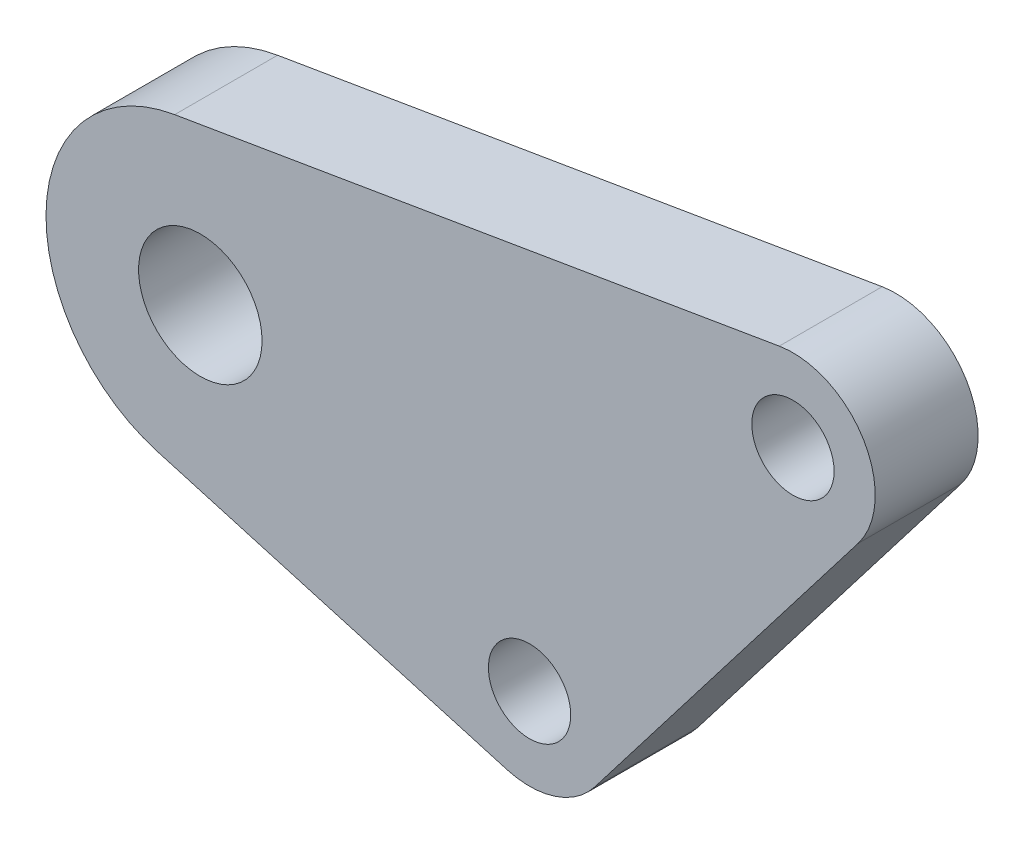
SolidWorks part; units mm, degrees
ref_plane "Front Plane" through (0, 0, 0) normal (0, 0, 1) x (1, 0, 0)
ref_plane "Top Plane" through (0, 0, 0) normal (0, 1, 0) x (1, 0, 0)
ref_plane "Right Plane" through (0, 0, 0) normal (1, 0, 0) x (0, 0, -1)
other "Configuration Table"
sketch "Sketch1" plane through (0, 0, 0) normal (0, 0, 1) x (1, 0, 0)
  line L0 (-17.2457, 15.6458) -> (12.1356, 20.5944)
  line L1 (15.9712, 14.2121) -> (3.1712, -2.4379)
  line L2 (-18.0755, 1.0429) -> (-1.107, -3.8438)
  circle A0 centre (0, 0) radius 2
  circle A1 centre (-16, 8.25) radius 3
  circle A2 centre (12.8, 16.65) radius 2
  arc A3 (-1.107, -3.8438) -> (3.1712, -2.4379) centre (0, 0) ccw
  arc A4 (15.9712, 14.2121) -> (12.1356, 20.5944) centre (12.8, 16.65) ccw
  arc A5 (-17.2457, 15.6458) -> (-18.0755, 1.0429) centre (-16, 8.25) ccw
  dimension "D1" = 4
  dimension "D2" = 4
  dimension "D3" = 6
  dimension "D8" = 15
  dimension "D9" = 8
  dimension "D10" = 8
  dimension "D4" = 16
  dimension "D5" = 12.8
  dimension "D6" = 8.25
  dimension "D7" = 8.4
extrude "Boss-Extrude1" add sketch "Sketch1" along normal blind 5
